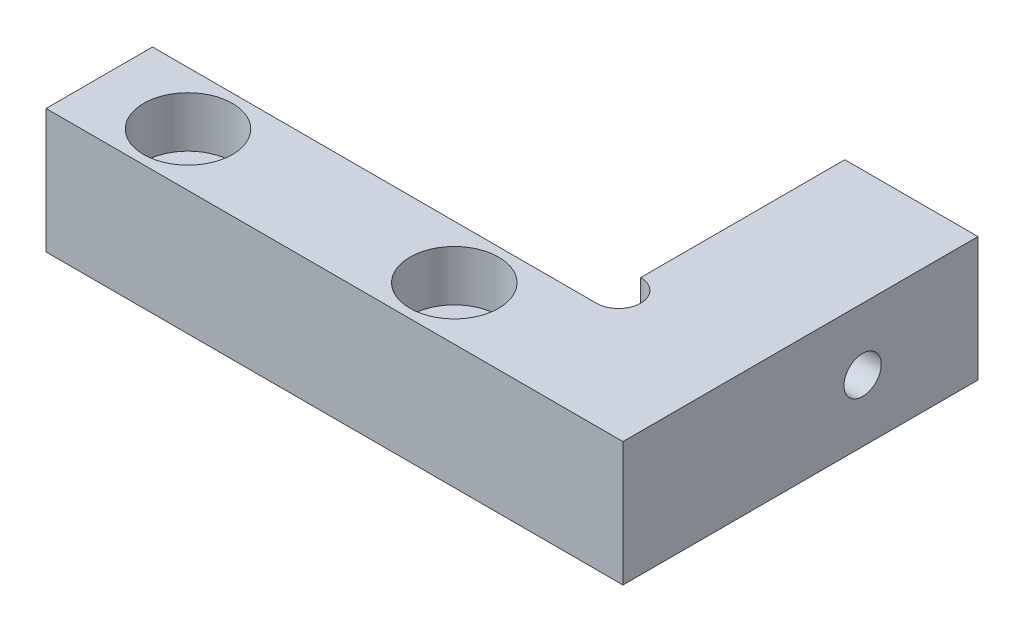
from build123d import *

# Parameters (mm, degrees)
SKETCH1_W                                           = 50
SKETCH1_H                                           = 12
BOSS_EXTRUDE1_DEPTH                                 = 7
HOLE_SIZE_PER_SOCKET_HEAD_CAP_SCREW_TYP_D           = 5.5
HOLE_SIZE_PER_SOCKET_HEAD_CAP_SCREW_TYP_CBORE_D     = 10
HOLE_SIZE_PER_SOCKET_HEAD_CAP_SCREW_TYP_CBORE_DEPTH = 5.7
SKETCH4_W                                           = 15
SKETCH4_H                                           = 40
BOSS_EXTRUDE2_DEPTH                                 = 14
M5_TAPPED_HOLE1_D                                   = 4.2
SKETCH8_R                                           = 2.5
CUT_EXTRUDE1_DEPTH                                  = 55.332310829


with BuildPart() as part:
    # Sketch1 → Boss-Extrude1 (new, symmetric)
    with BuildSketch(Plane(origin=(0, 0, 0), x_dir=(1, 0, 0), z_dir=(0, 1, 0))):
        Rectangle(SKETCH1_W, SKETCH1_H)
    extrude(amount=BOSS_EXTRUDE1_DEPTH, both=True)

    # Hole Size (per socket head cap screw type)1 (through all)
    with Locations(Plane(origin=(0, 7, 0), x_dir=(1, 0, 0), z_dir=(0, 1, 0))):
        with Locations((15, 0), (-15, 0)):
            CounterBoreHole(HOLE_SIZE_PER_SOCKET_HEAD_CAP_SCREW_TYP_D / 2, HOLE_SIZE_PER_SOCKET_HEAD_CAP_SCREW_TYP_CBORE_D / 2, HOLE_SIZE_PER_SOCKET_HEAD_CAP_SCREW_TYP_CBORE_DEPTH)

    # Sketch4 → Boss-Extrude2 (add)
    with BuildSketch(Plane(origin=(0, 7, 0), x_dir=(1, 0, 0), z_dir=(0, 1, 0))):
        with Locations((32.5, 14)):
            Rectangle(SKETCH4_W, SKETCH4_H)
    extrude(amount=-BOSS_EXTRUDE2_DEPTH)

    # M5 Tapped Hole1 (through all)
    with Locations(Plane(origin=(40, 0, 0), x_dir=(0, 0, -1), z_dir=(1, 0, 0))):
        with Locations((21, 0)):
            Hole(M5_TAPPED_HOLE1_D / 2)

    # Sketch8 → Cut-Extrude1 (cut, through all)
    with BuildSketch(Plane(origin=(0, 7, 0), x_dir=(1, 0, 0), z_dir=(0, 1, 0))):
        with Locations((25, 8.5)):
            Circle(SKETCH8_R)
    extrude(amount=-CUT_EXTRUDE1_DEPTH, mode=Mode.SUBTRACT)


solid = part.part
